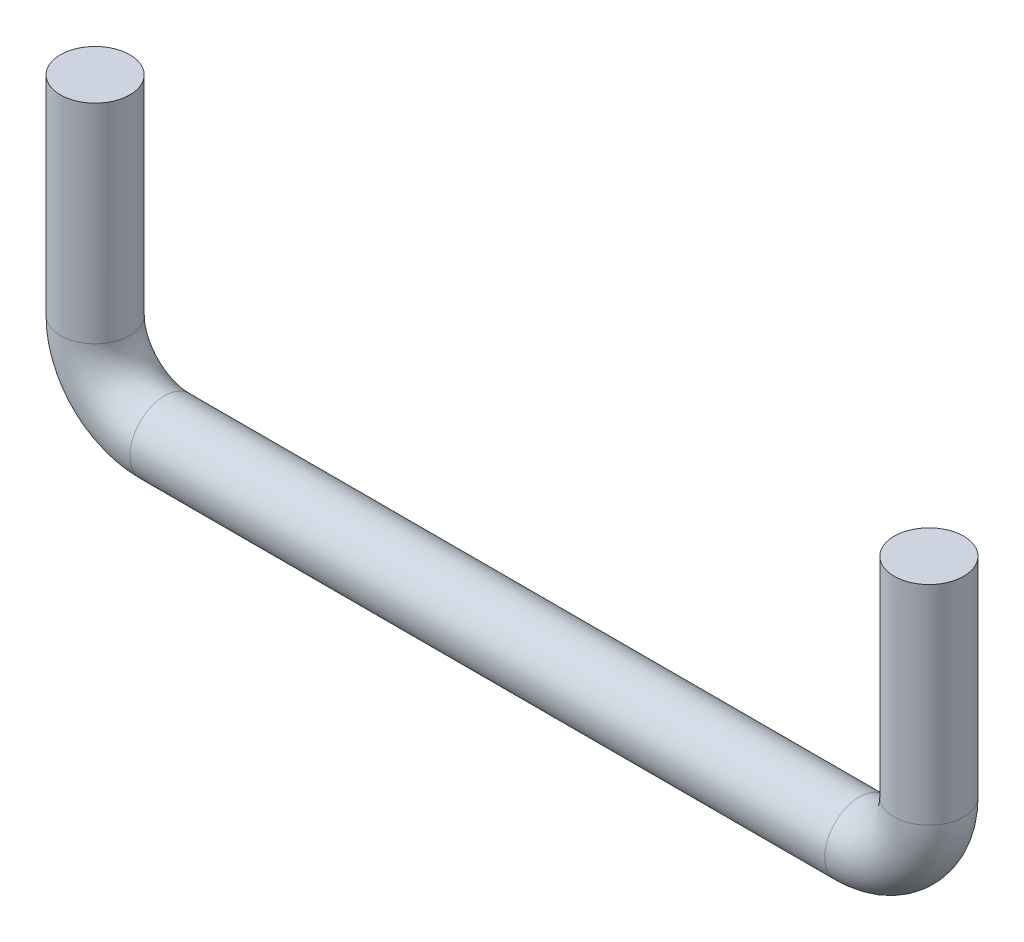
SolidWorks part; units mm, degrees
material "Q235A"
ref_plane "Front Plane" through (0, 0, 0) normal (0, 0, 1) x (1, 0, 0)
ref_plane "Top Plane" through (0, 0, 0) normal (0, 1, 0) x (1, 0, 0)
ref_plane "Right Plane" through (0, 0, 0) normal (1, 0, 0) x (0, 0, -1)
sketch "Sketch1" plane through (0, 0, 0) normal (0, 0, 1) x (1, 0, 0)
  line L0 (50, 0) -> (-50, 0)
  line L1 (-60, 10) -> (-60, 40)
  line L2 (60, 10) -> (60, 40)
  arc A0 (-60, 10) -> (-50, 0) centre (-50, 10) ccw
  arc A1 (50, 0) -> (60, 10) centre (50, 10) ccw
  point P4 (0, 0)
  point P9 (-60, 0)
  point P12 (60, 0)
  dimension "D3" = 10
  dimension "D1" = 120
  dimension "D2" = 40
sweep "Sweep1" add path "Sketch1" circular profile diameter 10 parameters "D3"=10
